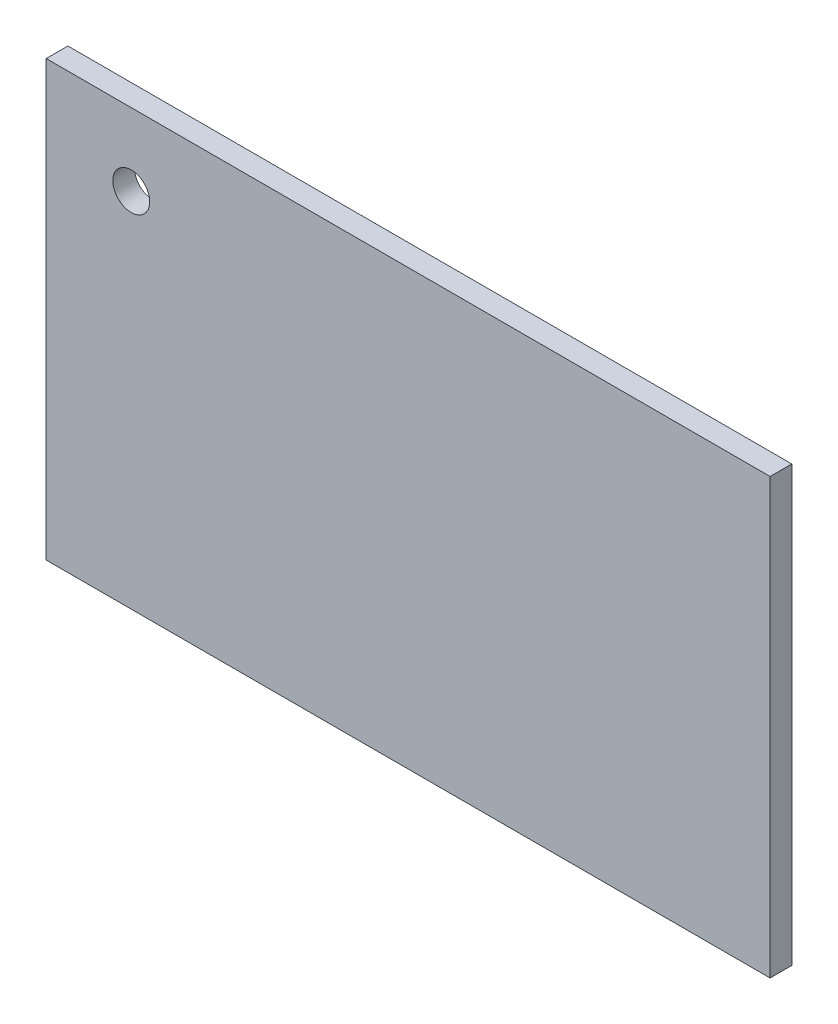
SolidWorks part; units mm, degrees
material "1023 碳钢板 (SS)"
ref_plane "Front Plane" through (0, 0, 0) normal (0, 0, 1) x (1, 0, 0)
ref_plane "Top Plane" through (0, 0, 0) normal (0, 1, 0) x (1, 0, 0)
ref_plane "Right Plane" through (0, 0, 0) normal (1, 0, 0) x (0, 0, -1)
sketch "Sketch1" plane through (0, 0, 0) normal (0, 0, 1) x (1, 0, 0)
  line L1 (100, 60) -> (-100, 60)
  line L2 (100, 60) -> (100, -60)
  line L3 (100, -60) -> (-100, -60)
  line L4 (-100, 60) -> (-100, -60)
  line L5 (100, 60) -> (-100, -60) construction
  line L6 (100, -60) -> (-100, 60) construction
  point P0 (0, 0)
  dimension "D1" = 200
  dimension "D2" = 120
extrude "Boss-Extrude1" add sketch "Sketch1" along normal blind 6
sketch "Sketch2" plane through (0, 0, 6) normal (0, 0, 1) x (1, 0, 0)
  line L0 (100, 60) -> (-100, 60) construction
  line L1 (-100, 60) -> (-100, -60) construction
  circle A0 centre (-76.5, 40) radius 5
  dimension "D1" = 10
  dimension "D3" = 10
  dimension "D4" = 23.5
  dimension "D2" = 20
hole_wizard "M12 Tapped Hole1" positions "Sketch3" profile "Sketch4" tap size "M12" standard "ISO"
sketch "Sketch3" plane through (0, 0, 6) normal (0, 0, 1) x (1, 0, 0)
  point P0 (-76.5, 40)
sketch "Sketch4" plane through (-76.5, 40, 6) normal (1, 0, 0) x (0, -1, 0)
  line L0 (0, 0) -> (0, 32.3144)
  line L1 (0, 32.3144) -> (5.1, 29.25)
  line L2 (5.1, 29.25) -> (5.1, 0)
  line L5 (5.1, 0) -> (0, 0)
  line L10 (0, 32.3144) -> (-5.1, 29.25) construction
  line L11 (0, -6.35) -> (0, 107.95) construction
  dimension "螺纹孔钻头直径" = 10.2
  dimension "螺纹孔钻头深度" = 29.25
  dimension "导头角度" = 118
cosmetic thread "Hole Thread Line 1"
